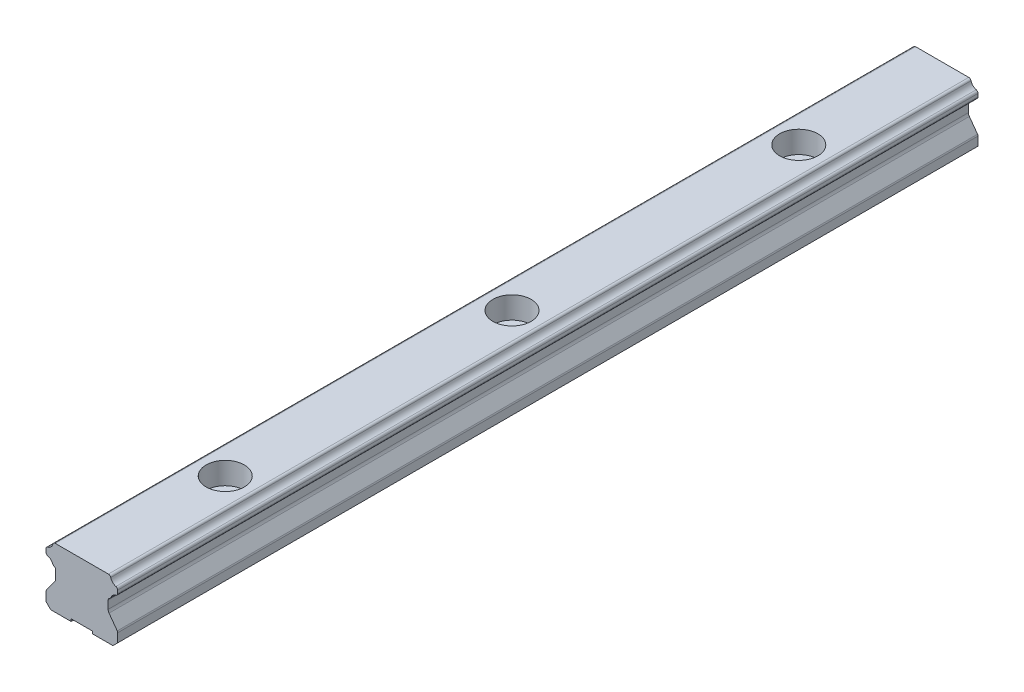
SolidWorks part; units mm, degrees
ref_plane "前视基准面" through (0, 0, 0) normal (0, 0, 1) x (1, 0, 0)
ref_plane "上视基准面" through (0, 0, 0) normal (0, 1, 0) x (1, 0, 0)
ref_plane "右视基准面" through (0, 0, 0) normal (1, 0, 0) x (0, 0, -1)
sketch "草图1" plane through (0, 0, 0) normal (0, 0, 1) x (1, 0, 0)
  line B0 (-7.5, -9.6626) -> (-7.5, -11.5)
  line B1 (-7.5, -11.5) -> (-6.5, -12.5)
  line B2 (-6.5, -12.5) -> (-2.25, -12.5)
  line B3 (-2.25, -12.5) -> (-2.25, -12)
  line B4 (-2.25, -12) -> (2.25, -12)
  line B5 (2.25, -12) -> (2.25, -12.5)
  line B6 (2.25, -12.5) -> (6.5, -12.5)
  line B7 (6.5, -12.5) -> (7.5, -11.5)
  line B8 (7.5, -11.5) -> (7.5, -9.6626)
  line B9 (7.4044, -9.3685) -> (5.6913, -7.013)
  line B10 (5.5, -6.4248) -> (5.5, -4.75)
  line B11 (5.7, -4.35) -> (5.9371, -4.1721)
  line B12 (7.5, -2.5635) -> (7.5, -1.9365)
  line B13 (5.5635, 0) -> (-5.5635, 0)
  line B14 (-7.5, -1.9365) -> (-7.5, -2.5635)
  line B15 (-5.9371, -4.1721) -> (-5.7, -4.35)
  line B16 (-5.5, -4.75) -> (-5.5, -6.4248)
  line B17 (-5.6913, -7.013) -> (-7.4044, -9.3685)
  arc B18 (7.5, -9.6626) -> (7.4044, -9.3685) centre (7, -9.6626) ccw
  arc B19 (5.5, -6.4248) -> (5.6913, -7.013) centre (6.5, -6.4248) ccw
  arc B20 (5.7, -4.35) -> (5.5, -4.75) centre (6, -4.75) ccw
  arc B21 (5.9371, -4.1721) -> (6.1029, -3.9541) centre (5.6371, -3.7721) ccw
  arc B22 (7.125, -3.0476) -> (6.1029, -3.9541) centre (7.5, -4.5) ccw
  arc B23 (7.125, -3.0476) -> (7.5, -2.5635) centre (7, -2.5635) ccw
  arc B24 (7.5, -1.9365) -> (7.125, -1.4524) centre (7, -1.9365) ccw
  arc B25 (6.0476, -0.375) -> (7.125, -1.4524) centre (7.5, 0) ccw
  arc B26 (6.0476, -0.375) -> (5.5635, 0) centre (5.5635, -0.5) ccw
  arc B27 (-5.5635, 0) -> (-6.0476, -0.375) centre (-5.5635, -0.5) ccw
  arc B28 (-7.125, -1.4524) -> (-6.0476, -0.375) centre (-7.5, 0) ccw
  arc B29 (-7.125, -1.4524) -> (-7.5, -1.9365) centre (-7, -1.9365) ccw
  arc B30 (-7.5, -2.5635) -> (-7.125, -3.0476) centre (-7, -2.5635) ccw
  arc B31 (-6.1029, -3.9541) -> (-7.125, -3.0476) centre (-7.5, -4.5) ccw
  arc B32 (-6.1029, -3.9541) -> (-5.9371, -4.1721) centre (-5.6371, -3.7721) ccw
  arc B33 (-5.5, -4.75) -> (-5.7, -4.35) centre (-6, -4.75) ccw
  arc B34 (-5.6913, -7.013) -> (-5.5, -6.4248) centre (-6.5, -6.4248) ccw
  arc B35 (-7.4044, -9.3685) -> (-7.5, -9.6626) centre (-7, -9.6626) ccw
sketch_block_instance "块1-1"
sketch_block "块1"
extrude "凸台-拉伸1" add sketch "草图1" along normal mid plane 180
hole_wizard "打孔尺寸(%根据)内六角圆柱头螺钉的类型1" positions "3D草图1" profile "草图2" counterbore size "M4" standard "GB" end condition up to next
sketch3d "3D草图1"
  line L0 (0, 0, -90) -> (0, 0, 90) construction
  line L1 (5.5635, 0, -90) -> (-5.5635, 0, -90) construction
  line L2 (5.5635, 0, 90) -> (-5.5635, 0, 90) construction
  point P0 (0, 0, -60)
  dimension "D1" = 30
sketch "草图2" plane through (0, 0, -60) normal (1, 0, 0) x (0, 0, 1)
  line L0 (0, 0) -> (0, 12.001)
  line L1 (0, 12.001) -> (2.25, 12.001)
  line L3 (2.25, 12.001) -> (2.25, 4.6)
  line L4 (2.25, 4.6) -> (4, 4.6)
  line L5 (4, 4.6) -> (4, 0)
  line L7 (4, 0) -> (0, 0)
  line L11 (0, -6.35) -> (0, 107.95) construction
  dimension "通孔孔直径" = 4.5
  dimension "通孔孔深度" = 12.001
  dimension "柱形沉头孔直径" = 8
  dimension "柱形沉头孔深度" = 4.6
pattern_linear "阵列(线性)2" count 3 spacing 60 along (0, 0, 1) of "打孔尺寸(%根据)内六角圆柱头螺钉的类型1"
